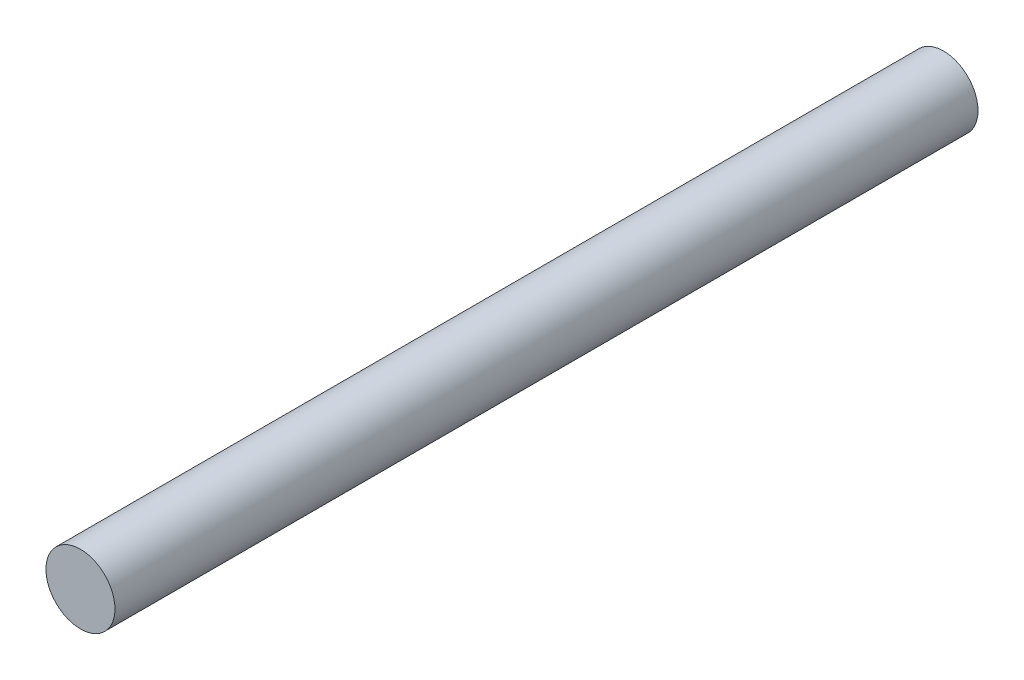
SolidWorks part; units mm, degrees
ref_plane "Front" through (0, 0, 0) normal (0, 0, 1) x (1, 0, 0)
ref_plane "Top" through (0, 0, 0) normal (0, 1, 0) x (1, 0, 0)
ref_plane "Right" through (0, 0, 0) normal (1, 0, 0) x (0, 0, -1)
sketch "Sketch1" plane through (0, 0, 0) normal (0, 0, 1) x (1, 0, 0)
  circle A0 centre (0, 0) radius 20
extrude "Boss-Extrude1" add sketch "Sketch1" along normal blind 500
